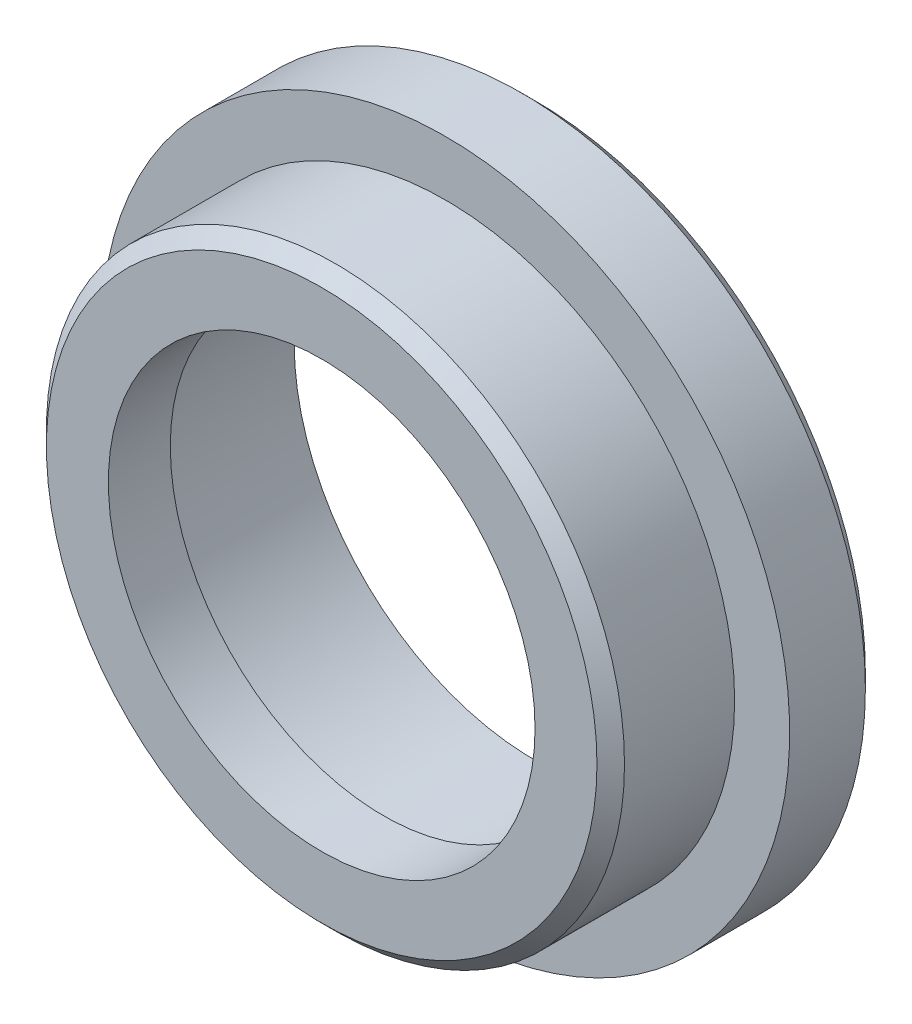
SolidWorks part; units mm, degrees
ref_plane "Front Plane" through (0, 0, 0) normal (0, 0, 1) x (1, 0, 0)
ref_plane "Top Plane" through (0, 0, 0) normal (0, 1, 0) x (1, 0, 0)
ref_plane "Right Plane" through (0, 0, 0) normal (1, 0, 0) x (0, 0, -1)
other "Configuration Table"
sketch "Sketch1" plane through (0, 0, 0) normal (0, 0, 1) x (1, 0, 0)
  circle A0 centre (0, 0) radius 25
  dimension "D1" = 50
extrude "Boss-Extrude1" add sketch "Sketch1" along normal blind 6.5
sketch "Sketch2" plane through (0, 0, 6.5) normal (0, 0, 1) x (1, 0, 0)
  circle A0 centre (0, 0) radius 21
  dimension "D1" = 42
extrude "Boss-Extrude3" add sketch "Sketch2" along normal blind 9
sketch "Sketch5" plane through (0, 0, 15.5) normal (0, 0, 1) x (1, 0, 0)
  circle A0 centre (0, 0) radius 15.5
  dimension "D1" = 31
extrude "Cut-Extrude2" cut sketch "Sketch5" against normal blind 43
sketch "Sketch6" plane through (0, 0, 0) normal (0, 0, -1) x (-1, 0, 0)
  circle A0 centre (0, 0) radius 17.5
  dimension "D1" = 35
extrude "Cut-Extrude3" cut sketch "Sketch6" against normal blind 11
sketch "Sketch7" plane through (0, 0, 11) normal (0, 0, -1) x (-1, 0, 0)
  circle A0 centre (0, 0) radius 16.5
  circle A1 centre (0, 0) radius 17.5
  dimension "D1" = 33
  dimension "D2" = 35
extrude "Cut-Extrude4" cut sketch "Sketch7" against normal blind 0.5
chamfer "Chamfer1" distance 1 angle 45 2 edges at (21, 0, 15.5) (25, 0, 0)
